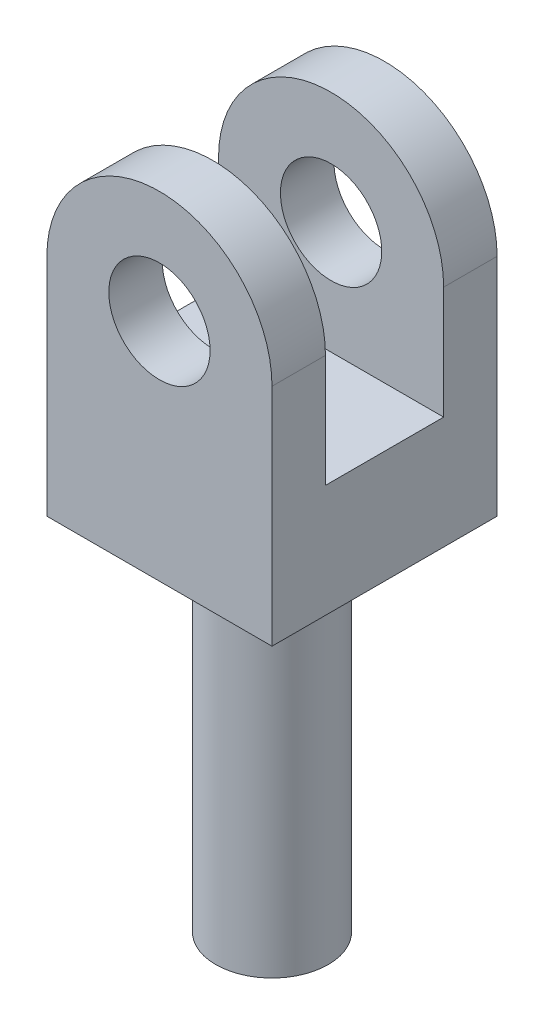
SolidWorks part; units mm, degrees
material "Q235B"
ref_plane "Front Plane" through (0, 0, 0) normal (0, 0, 1) x (1, 0, 0)
ref_plane "Top Plane" through (0, 0, 0) normal (0, 1, 0) x (1, 0, 0)
ref_plane "Right Plane" through (0, 0, 0) normal (1, 0, 0) x (0, 0, -1)
sketch "Sketch1" plane through (0, 0, 0) normal (0, 0, 1) x (1, 0, 0)
  line L1 (140.4025, -159.5975) -> (-59.5975, -159.5975)
  line L2 (140.4025, -159.5975) -> (140.4025, 40.4025)
  line L3 (140.4025, 40.4025) -> (-59.5975, 40.4025) construction
  line L4 (-59.5975, -159.5975) -> (-59.5975, 40.4025)
  line L5 (140.4025, -159.5975) -> (-59.5975, 40.4025) construction
  line L6 (140.4025, 40.4025) -> (-59.5975, -159.5975) construction
  arc A0 (140.4025, 40.4025) -> (-59.5975, 40.4025) centre (40.4025, 40.4025) ccw
  circle A1 centre (40.4025, 40.4025) radius 45
  point P0 (40.4025, -59.5975)
  dimension "D1" = 90
  dimension "D2" = 100
extrude "Boss-Extrude2" add sketch "Sketch1" along normal blind 200
sketch "Sketch2" plane through (140.4025, 0, 0) normal (1, 0, 0) x (0, 0, -1)
  line L0 (-100, 140.4025) -> (-100, -159.5975) construction
  line L1 (0, 140.4025) -> (-200, 140.4025) construction
  line L2 (-200, -159.5975) -> (0, -159.5975) construction
  line L4 (-152.5, 258.4524) -> (-47.5, 258.4524)
  line L5 (-152.5, 258.4524) -> (-152.5, -59.5975)
  line L6 (-152.5, -59.5975) -> (-47.5, -59.5975)
  line L7 (-47.5, 258.4524) -> (-47.5, -59.5975)
  line L8 (-152.5, 258.4524) -> (-47.5, -59.5975) construction
  line L9 (-152.5, -59.5975) -> (-47.5, 258.4524) construction
  point P6 (-100, 99.4274)
  dimension "D2" = 100
  dimension "D3" = 105
extrude "Cut-Extrude1" cut sketch "Sketch2" against normal through all
sketch "Sketch3" plane through (0, -159.5975, 0) normal (0, -1, 0) x (1, 0, 0)
  line L0 (40.4025, 200) -> (40.4025, 0) construction
  line L1 (-59.5975, 200) -> (140.4025, 200) construction
  line L2 (-59.5975, 0) -> (140.4025, 0) construction
  circle A0 centre (40.4025, 100) radius 50
  dimension "D1" = 100
extrude "Boss-Extrude3" add sketch "Sketch3" along normal blind 320
sketch "Sketch4" plane through (0, -479.5975, 0) normal (0, -1, 0) x (1, 0, 0)
  circle A0 centre (40.4025, 100) radius 25
  dimension "D1" = 50
extrude "Cut-Extrude2" cut sketch "Sketch4" against normal blind 100
fillet "Fillet1" radius 10 1 edges at (90.4025, -159.5975, 100)
equation "\"dhgs\"= \"代号公式\""
equation "\"mcgs\"= \"名称公式\""
